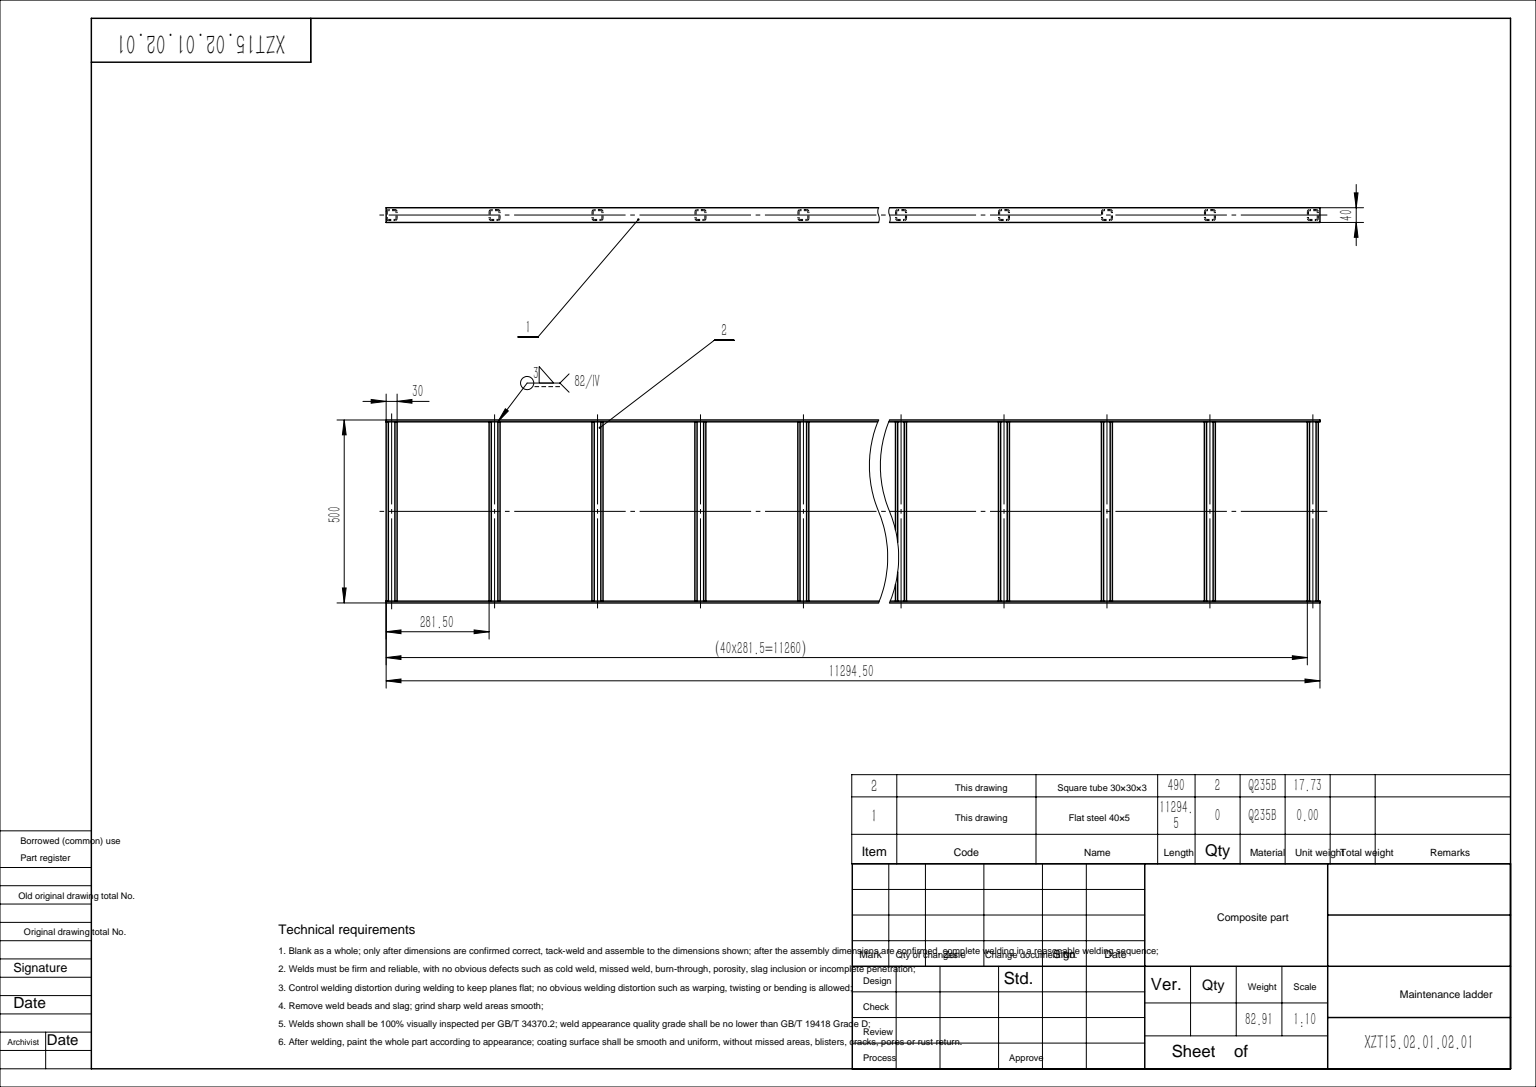
SolidWorks part; units mm, degrees
material "Q235B"
ref_plane "Front Plane" through (0, 0, 0) normal (0, 0, 1) x (1, 0, 0)
ref_plane "Top Plane" through (0, 0, 0) normal (0, 1, 0) x (1, 0, 0)
ref_plane "Right Plane" through (0, 0, 0) normal (1, 0, 0) x (0, 0, -1)
sketch "草图1" plane through (0, 0, 0) normal (0, 0, 1) x (1, 0, 0)
  line L0 (-20, 0) -> (-20, 100.1568)
  line L1 (-19.7676, 101.8106) -> (2.3661, 179)
  line L2 (0, 20) -> (-13.95, 20)
  arc A0 (-20, 0) -> (0, 20) centre (0, 0) ccw
  arc A1 (-20, 100.1568) -> (-19.7676, 101.8106) centre (-14, 100.1568) cw
  point P9 (-20, 101)
  dimension "D1" = 40
  dimension "D6" = 6
  dimension "D2" = 101
  dimension "D3" = 164
  dimension "D4" = 78
  dimension "D5" = 6.05
sweep "Sweep2" add path "草图1" circular profile diameter 12 parameters "D3"=12
chamfer "Chamfer1" distance 0.5 angle 45 1 edges at (-3.4014, 180.6538, 0)
sketch "Sketch2" plane through (0, 0, 0) normal (0, 0, 1) x (1, 0, 0)
  line L0 (56.1154, 366.446) -> (-425.4767, 504.5403) construction
  line L3 (-3062.8383, -10488.8704) -> (50.3479, 368.0999)
  line L4 (-3.5392, 180.1732) -> (-25.5351, 103.4644) construction
  line L5 (-425.4767, 504.5403) -> (-3538.6628, -10352.4299)
  line L6 (-3534.5282, -10338.011) -> (-3058.7037, -10474.4514)
  line L7 (-3456.9363, -10067.4158) -> (-2981.1118, -10203.8563)
  line L8 (2.3661, 179) -> (56.1154, 366.446)
  line L9 (7.6531, 177.484) -> (-2.9208, 180.516) construction
  dimension "D1" = 11294.5
  dimension "D2" = 495
  dimension "D3" = 15
  dimension "D4" = 281.5
  dimension "D5" = 195
ref_plane "Plane2" through (0, 0, -20) normal (0, 0, 1) x (1, 0, 0)
sketch "Sketch7" plane through (0, 0, -20) normal (0, 0, 1) x (1, 0, 0)
  line L0 (-3456.9363, -10067.4158) -> (-2981.1118, -10203.8563) construction
  line L1 (-3534.5282, -10338.011) -> (-3058.7037, -10474.4514) construction
  line L2 (-425.4767, 504.5403) -> (-3538.6628, -10352.4299) construction
  line L3 (-3062.8383, -10488.8704) -> (50.3479, 368.0999) construction
  line L4 (-3456.9363, -10067.4158) -> (-2981.1118, -10203.8563)
  line L5 (-3534.5282, -10338.011) -> (-3058.7037, -10474.4514)
  line L6 (-425.4767, 504.5403) -> (-3538.6628, -10352.4299)
  line L7 (-3062.8383, -10488.8704) -> (50.3479, 368.0999)
other "GB/T 704-1988 hot-rolled flat steel 40×5(1)"
ref_plane "Plane3" through (-3062.8383, -10488.8704, -20) normal (-0.2756, -0.9613, 0) x (0, 0, 1)
sketch "Sketch14" plane through (-3062.8383, -10488.8704, -20) normal (-0.2756, -0.9613, 0) x (0, 0, 1)
  line L0 (0, 0) -> (0, 5)
  line L1 (40, 0) -> (40, 5)
  line L3 (0, 5) -> (40, 5)
  line L4 (20, 5) -> (20, 0) construction
  line L5 (40, 0) -> (0, 0)
  point P1 (0, 0)
  point P10 (20, 0)
  point P16 (20, 5)
  point P18 (40, 5)
  dimension "D3" = 40
  dimension "D1" = 5
other "GB/T 6728-2002 square hollow section 30×3-example.com(1)"
ref_plane "Plane5" through (-3534.5282, -10338.011, 0) normal (0.9613, -0.2756, 0) x (0.2756, 0.9613, 0)
sketch "Sketch1" plane through (-3534.5282, -10338.011, 0) normal (0.9613, -0.2756, 0) x (0.2756, 0.9613, 0)
  line L0 (-9, -12) -> (9, -12)
  line L1 (-12, -9) -> (-12, 9)
  line L2 (9, 12) -> (-9, 12)
  line L3 (12, 9) -> (12, -9)
  line L4 (-9, -15) -> (9, -15)
  line L5 (-15, -9) -> (-15, 9)
  line L6 (9, 15) -> (-9, 15)
  line L7 (15, 9) -> (15, -9)
  arc A0 (15, 9) -> (9, 15) centre (9, 9) ccw
  arc A1 (9, -15) -> (15, -9) centre (9, -9) ccw
  arc A2 (-15, -9) -> (-9, -15) centre (-9, -9) ccw
  arc A3 (-9, 15) -> (-15, 9) centre (-9, 9) ccw
  arc A4 (-9, 12) -> (-12, 9) centre (-9, 9) ccw
  arc A5 (12, 9) -> (9, 12) centre (9, 9) ccw
  arc A6 (9, -12) -> (12, -9) centre (9, -9) ccw
  arc A7 (-12, -9) -> (-9, -12) centre (-9, -9) ccw
  point P0 (-15, 0)
  point P1 (15, 0)
  point P2 (0, 15)
  point P3 (0, -15)
  point P4 (0, 0)
  point P5 (-15, -15)
  point P6 (15, -15)
  point P7 (15, 15)
  point P8 (-15, 15)
  point P33 (0, 0)
  dimension "D1" = 6
  dimension "Thickness" = 3
  dimension "V_leg" = 30
other "Trim/Extend1"
pattern_linear "LinearPattern1" count 40 spacing 281.5 along (0.2756, 0.9613, 0) of bodies 113
sketch "Sketch10" plane through (0, 0, 20) normal (0, 0, 1) x (1, 0, 0)
  line L0 (2.9464, 202.7913) -> (-74.4749, -67.2087)
  line L1 (2.9464, 202.7913) -> (117.9464, 169.8156)
  line L2 (-74.4749, -67.2087) -> (40.5251, -100.1844)
  line L3 (117.9464, 169.8156) -> (40.5251, -100.1844)
  line L4 (50.3479, 368.0999) -> (-3062.8383, -10488.8704) construction
  dimension "D1" = 115
  dimension "D2" = 270
extrude "Cut-Extrude1" cut sketch "Sketch10" against normal through all both and the other way through all
